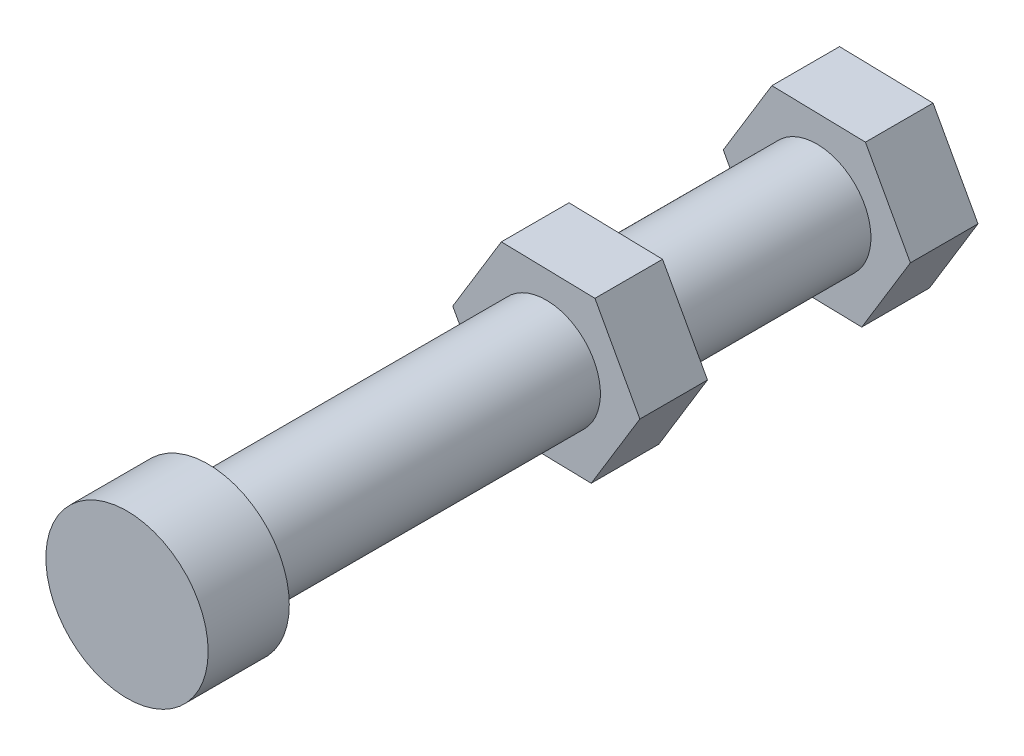
from build123d import *

# Parameters (mm, degrees)
SKETCH1_R           = 4
BOSS_EXTRUDE1_DEPTH = 50
SKETCH2_R           = 6
BOSS_EXTRUDE2_DEPTH = 6
BOSS_EXTRUDE3_DEPTH = 5
LPATTERN1_COUNT     = 2
LPATTERN1_PITCH     = 20


with BuildPart() as part:
    # Sketch1 → Boss-Extrude1 (new body)
    with BuildSketch(Plane.XY):
        Circle(SKETCH1_R)
    extrude(amount=BOSS_EXTRUDE1_DEPTH)

    # Sketch2 → Boss-Extrude2 (add)
    with BuildSketch(Plane.XY.offset(50)):
        Circle(SKETCH2_R)
    extrude(amount=BOSS_EXTRUDE2_DEPTH)

    # Sketch3 → Boss-Extrude3 (add)
    with BuildSketch(Plane(origin=(0, 0, 0), x_dir=(-1, 0, 0), z_dir=(0, 0, -1))):
        Polygon((3.321586055, 6.06931697), (-3.595389652, 5.911236389), (-6.916975707, -0.158080581), (-3.321586055, -6.06931697), (3.595389652, -5.911236389), (6.916975707, 0.158080581), align=None)
    boss_extrude3 = extrude(amount=-BOSS_EXTRUDE3_DEPTH)

    # LPattern1: Boss-Extrude3 ×2
    with Locations(*[(0, 0, i * LPATTERN1_PITCH) for i in range(1, LPATTERN1_COUNT)]):
        add(boss_extrude3)


solid = part.part
